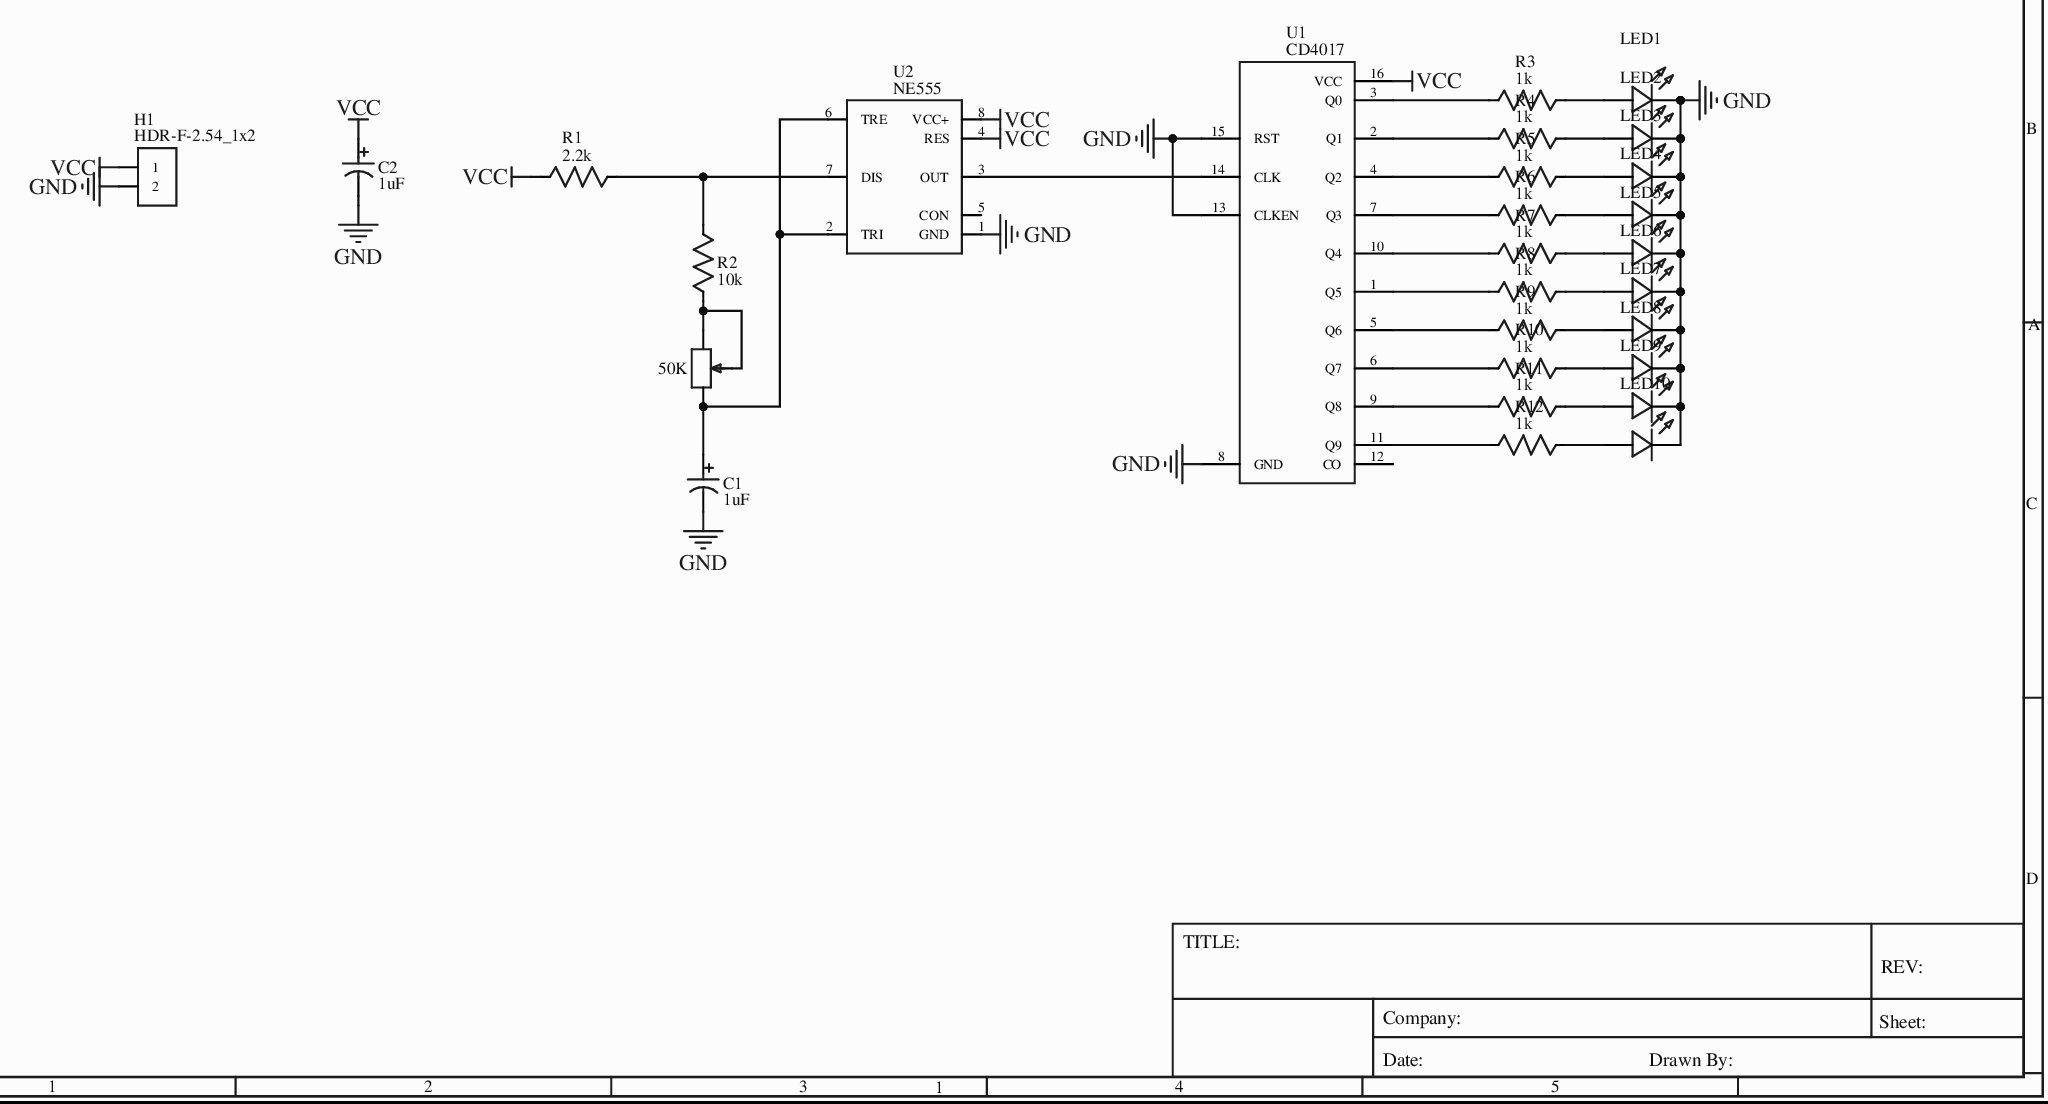
[diagram p0: MISC49871-2.schdoc]
# Altium project MISC49871.PrjPcb
1 sheet, 28 parts. Net scope: global (net labels, ports and power ports of the same name join across sheets).
Board file: MISC49871.pcbdoc

## Sheet MISC49871-2.schdoc
size 292 x 204 mm; Name: MISC49871; @Project Name: MISC49871

### Parts
C1  1uF  [CAP-TH_BD5.0-P2.00-D0.8-FD]
C2  1uF  [CAP-TH_BD5.0-P2.00-D0.8-FD]
H1  HDR-F-2.54_1x2  [HDR-F-2.54_1X2]
LED1  LED-TH-3mm_R  [LED-TH_BD3.0_RED]  (value not drawn)
LED2  LED-TH-3mm_R  [LED-TH_BD3.0_RED]  (value not drawn)
LED3  LED-TH-3mm_R  [LED-TH_BD3.0_RED]  (value not drawn)
LED4  LED-TH-3mm_R  [LED-TH_BD3.0_RED]  (value not drawn)
LED5  LED-TH-3mm_R  [LED-TH_BD3.0_RED]  (value not drawn)
LED6  LED-TH-3mm_R  [LED-TH_BD3.0_RED]  (value not drawn)
LED7  LED-TH-3mm_R  [LED-TH_BD3.0_RED]  (value not drawn)
LED8  LED-TH-3mm_R  [LED-TH_BD3.0_RED]  (value not drawn)
LED9  LED-TH-3mm_R  [LED-TH_BD3.0_RED]  (value not drawn)
LED10  LED-TH-3mm_R  [LED-TH_BD3.0_RED]  (value not drawn)
R1  2.2k  [R_AXIAL-0.4]
R2  10k  [R_AXIAL-0.4]
R3  1k  [R_AXIAL-0.4]
R4  1k  [R_AXIAL-0.4]
R5  1k  [R_AXIAL-0.4]
R6  1k  [R_AXIAL-0.4]
R7  1k  [R_AXIAL-0.4]
R8  1k  [R_AXIAL-0.4]
R9  1k  [R_AXIAL-0.4]
R10  1k  [R_AXIAL-0.4]
R11  1k  [R_AXIAL-0.4]
R12  1k  [R_AXIAL-0.4]
R13  50K  [RES-ADJ-SMD_RM065-V1]
U1  CD4017  [CD4017]
U2  NE555  [DIP08-KIT]

### Nets
GND: C1.2 C2.2 H1.2 LED1.2 LED2.2 LED3.2 LED4.2 LED5.2 LED6.2 LED7.2 LED8.2 LED9.2 LED10.2 U1.8(GND) U1.13(CLKEN) U1.15(RST) U2.1(GND)
VCC: C2.1 H1.1 R1.2 U1.16(VCC) U2.4(RES) U2.8(VCC+)
NetC1_1: C1.1 R13.3 U2.2(TRI) U2.6(TRE)
NetLED1_1: LED1.1 R3.2
NetLED2_1: LED2.1 R4.2
NetLED3_1: LED3.1 R5.2
NetLED4_1: LED4.1 R6.2
NetLED5_1: LED5.1 R7.2
NetLED6_1: LED6.1 R8.2
NetLED7_1: LED7.1 R9.2
NetLED8_1: LED8.1 R10.2
NetLED9_1: LED9.1 R11.2
NetLED10_1: LED10.1 R12.2
NetR1_1: R1.1 R2.2 U2.7(DIS)
NetR2_1: R2.1 R13.1 R13.2
NetR3_1: R3.1 U1.3(Q0)
NetR4_1: R4.1 U1.2(Q1)
NetR5_1: R5.1 U1.4(Q2)
NetR6_1: R6.1 U1.7(Q3)
NetR7_1: R7.1 U1.10(Q4)
NetR8_1: R8.1 U1.1(Q5)
NetR9_1: R9.1 U1.5(Q6)
NetR10_1: R10.1 U1.6(Q7)
NetR11_1: R11.1 U1.9(Q8)
NetR12_1: R12.1 U1.11(Q9)
NetU1_14: U1.14(CLK) U2.3(OUT)

Not connected (* = marked no-connect by the designer): U1 12(CO)*; U2 5(CON)*

### Notes on the sheet
- 1
- 2
- 3
- 4
- 5
- A
- B
- C
- D
- TITLE:
- Company:
- Sheet:
- REV:
- Date:
- Drawn By:

### Library data of the parts
C1 C2 = 1uF 50V 5*11: Manufacturer: ValuePro; Convert to PCB: yes; Origin Footprint: CAP-TH_BD5.0-P2.00-D0.8-FD; Device: 1uF 50V 5*11; Symbol: 1uF; Add into BOM: yes; Supplier: LCSC; ManufacturerPart: 1uF 50V 5*11; SupplierPart: C43342; JLCPCB Part Class: Extended Part; FootprintName: CAP-TH_BD5.0-P2.00-D0.8-FD
H1 = HDR-F-2.54_1x2: Convert to PCB: yes; Origin Footprint: HDR-F-2.54_1X2; Device: HDR-F-2.54_1x2; Symbol: HDR-F-2.54_1x2; Add into BOM: yes; SupplierPart: C49661; Supplier: LCSC; FootprintName: HDR-F-2.54_1X2
LED1-LED10 = 204-10SDRD/S530-A3-L: Manufacturer: EVERLIGHT(台湾亿光); Convert to PCB: yes; Origin Footprint: LED-TH_BD3.0_RED; Device: 204-10SDRD/S530-A3-L; Symbol: LED-TH-3mm_R; Add into BOM: yes; ManufacturerPart: 204-10SDRD/S530-A3-L; SupplierPart: C84774; Supplier: LCSC; FootprintName: LED-TH_BD3.0_RED
R1 = 2.2k: Convert to PCB: yes; Origin Footprint: R_AXIAL-0.4; Device: 2.2k; Symbol: 2.2k; Add into BOM: yes; FootprintName: R_AXIAL-0.4
R2 = 10k: Convert to PCB: yes; Origin Footprint: R_AXIAL-0.4; Device: 10k; Symbol: 10k; Add into BOM: yes; FootprintName: R_AXIAL-0.4
R3-R12 = 1k: Convert to PCB: yes; Origin Footprint: R_AXIAL-0.4; Device: 1k; Symbol: 1k; Add into BOM: yes; FootprintName: R_AXIAL-0.4
R13 = RM065-V1-5K blue: Manufacturer: ReliaPro; Convert to PCB: yes; Origin Footprint: RES-ADJ-SMD_RM065-V1; Device: RM065-V1-5K blue; Symbol: 50K; Add into BOM: yes; Supplier: LCSC; ManufacturerPart: RM065-V1-5K blue; SupplierPart: C36862; JLCPCB Part Class: Extended Part; FootprintName: RES-ADJ-SMD_RM065-V1
U1 = CD4017SOIC: Convert to PCB: yes; Origin Footprint: CD4017; Device: CD4017SOIC; Symbol: CD4017; Add into BOM: yes; ManufacturerPart: CD4017SOIC; FootprintName: CD4017
U2 = NE555: Convert to PCB: yes; Origin Footprint: DIP08-KIT; Device: NE555; Symbol: NE555; Add into BOM: yes; FootprintName: DIP08-KIT